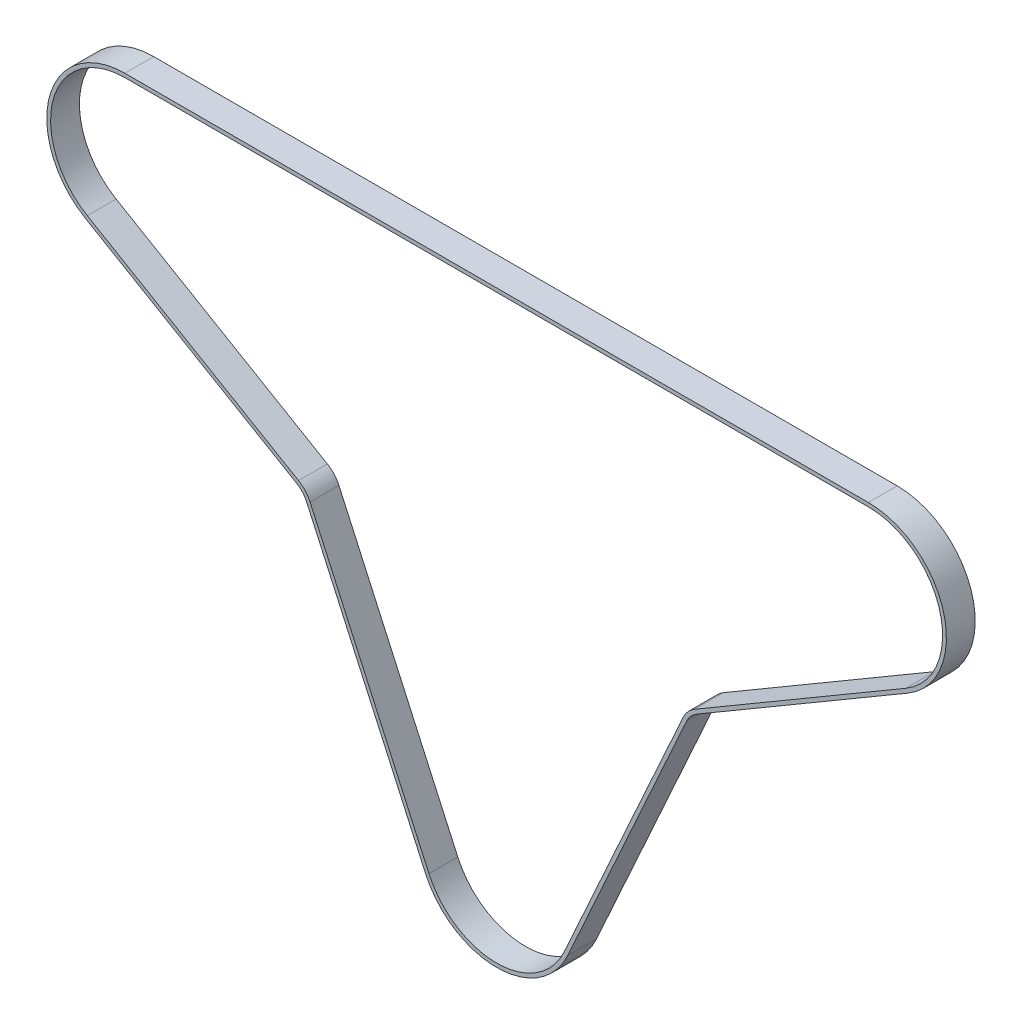
from build123d import *

# Parameters (mm, degrees)
EXTRUDE_1_DEPTH = 19


with BuildPart() as part:
    # 草图2 → 拉伸-薄壁1 (new, symmetric)
    with BuildSketch(Plane.XY):
        with BuildLine():
            Line((250.396106976, 303.41117138), (93.71226198, -42.453604657))
            ThreePointArc((93.71226198, -42.453604657), (0, -102.880025838), (-93.71226198, -42.453604657))
            Line((-93.71226198, -42.453604657), (-250.396106976, 303.41117138))
            ThreePointArc((-250.396106976, 303.41117138), (-255.84721668, 311.74610443), (-263.566360338, 318.038999402))
            Line((-263.566360338, 318.038999402), (-542.021317698, 481.241272274))
            ThreePointArc((-542.021317698, 481.241272274), (-589.286886818, 596.95176731), (-489.999999284, 672.879803303))
            Line((-489.999999284, 672.879803303), (490.000000716, 672.879803303))
            ThreePointArc((490.000000716, 672.879803303), (589.28688828, 596.951767199), (542.021318931, 481.241272157))
            Line((542.021318931, 481.241272157), (263.566360401, 318.038999439))
            ThreePointArc((263.566360401, 318.038999439), (255.847216704, 311.746104457), (250.396106976, 303.41117138))
        make_face()
        with BuildLine():
            Line((245.841661895, 305.474428516), (89.1578169, -40.390347521))
            ThreePointArc((89.1578169, -40.390347521), (0, -97.880025838), (-89.1578169, -40.390347521))
            Line((-89.1578169, -40.390347521), (-245.841661895, 305.474428516))
            ThreePointArc((-245.841661895, 305.474428516), (-252.131403861, 315.091658958), (-261.038108082, 322.352691617))
            Line((-261.038108082, 322.352691617), (-539.493065442, 485.554964489))
            ThreePointArc((-539.493065442, 485.554964489), (-584.461513202, 595.641893476), (-489.999999284, 667.879803303))
            Line((-489.999999284, 667.879803303), (490.000000716, 667.879803303))
            ThreePointArc((490.000000716, 667.879803303), (584.461514662, 595.641893371), (539.493066685, 485.554964378))
            Line((539.493066685, 485.554964378), (261.038108155, 322.35269166))
            ThreePointArc((261.038108155, 322.35269166), (252.131403889, 315.091658989), (245.841661895, 305.474428516))
        make_face(mode=Mode.SUBTRACT)
    extrude(amount=EXTRUDE_1_DEPTH, both=True)


solid = part.part
